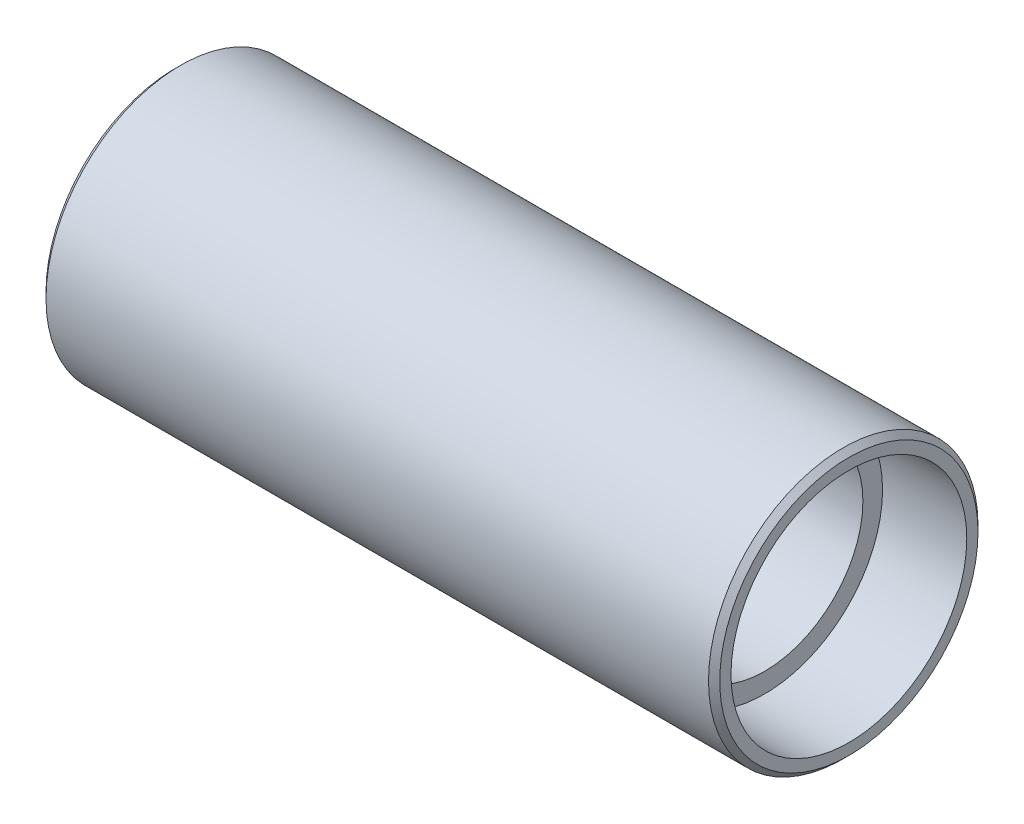
SolidWorks part; units mm, degrees
material "Q235"
ref_plane "Front Plane" through (0, 0, 0) normal (0, 0, 1) x (1, 0, 0)
ref_plane "Top Plane" through (0, 0, 0) normal (0, 1, 0) x (1, 0, 0)
ref_plane "Right Plane" through (0, 0, 0) normal (1, 0, 0) x (0, 0, -1)
sketch "Sketch1" plane through (0, 0, 0) normal (0, 0, 1) x (1, 0, 0)
  line L0 (0, 0) -> (0, 30)
  line L1 (0, 30) -> (120, 30)
  line L2 (120, 30) -> (120, 0)
  line L3 (120, 0) -> (0, 0)
  line L4 (0, 0) -> (-23.3371, 0) construction
  dimension "D1" = 120
  dimension "D2" = 60
revolve "Revolve1" add sketch "Sketch1" angle 360 about L4
sketch "Sketch2" plane through (0, 0, 0) normal (-1, 0, 0) x (0, 0, 1)
  circle A0 centre (0, 0) radius 21
  dimension "D1" = 42
extrude "Cut-Extrude1" cut sketch "Sketch2" against normal blind 15
sketch "Sketch4" plane through (120, 0, 0) normal (1, 0, 0) x (0, 0, -1)
  circle A1 centre (0, 0) radius 21
  circle A2 centre (0, 0) radius 21
  dimension "D1" = 0
extrude "Cut-Extrude2" cut sketch "Sketch4" against normal blind 15
sketch "Sketch5" plane through (105, 0, 0) normal (1, 0, 0) x (0, 0, -1)
  circle A0 centre (0, 0) radius 17.5
  dimension "D1" = 35
extrude "Cut-Extrude3" cut sketch "Sketch5" against normal through all
sketch "Sketch6" plane through (0, 0, 0) normal (0, 0, 1) x (1, 0, 0)
  line L0 (0, 29.65) -> (59.5, 30)
  line L1 (0, 30) -> (0, -30) construction
  line L2 (59.5, 30) -> (0, 30)
  line L3 (0, 30) -> (0, 29.65)
  line L4 (60, 30) -> (60, 16.6363) construction
  line L5 (120, 30) -> (0, 30) construction
  line L6 (120, 30) -> (120, 29.65)
  line L7 (60.5, 30) -> (120, 30)
  line L8 (120, 29.65) -> (60.5, 30)
  line L9 (0, 0) -> (15.5285, 0) construction
  dimension "D1" = 0.35
  dimension "D2" = 1
revolve "Cut-Revolve1" [suppressed] cut sketch "Sketch6" angle 360 about L9
sketch "Sketch8" plane through (0, 0, 0) normal (-1, 0, 0) x (0, 0, 1)
  circle A0 centre (0, 0) radius 41.444
  circle A1 centre (0, 0) radius 24
  dimension "D1" = 48
extrude "Cut-Extrude4" cut sketch "Sketch8" against normal through all
chamfer "Chamfer1" distance 1 angle 45 1 edges at (0, 0, 24)
chamfer "Chamfer2" [suppressed] distance 10 angle 6
chamfer "Chamfer3" distance 1 angle 45 1 edges at (120, 0, 24)
